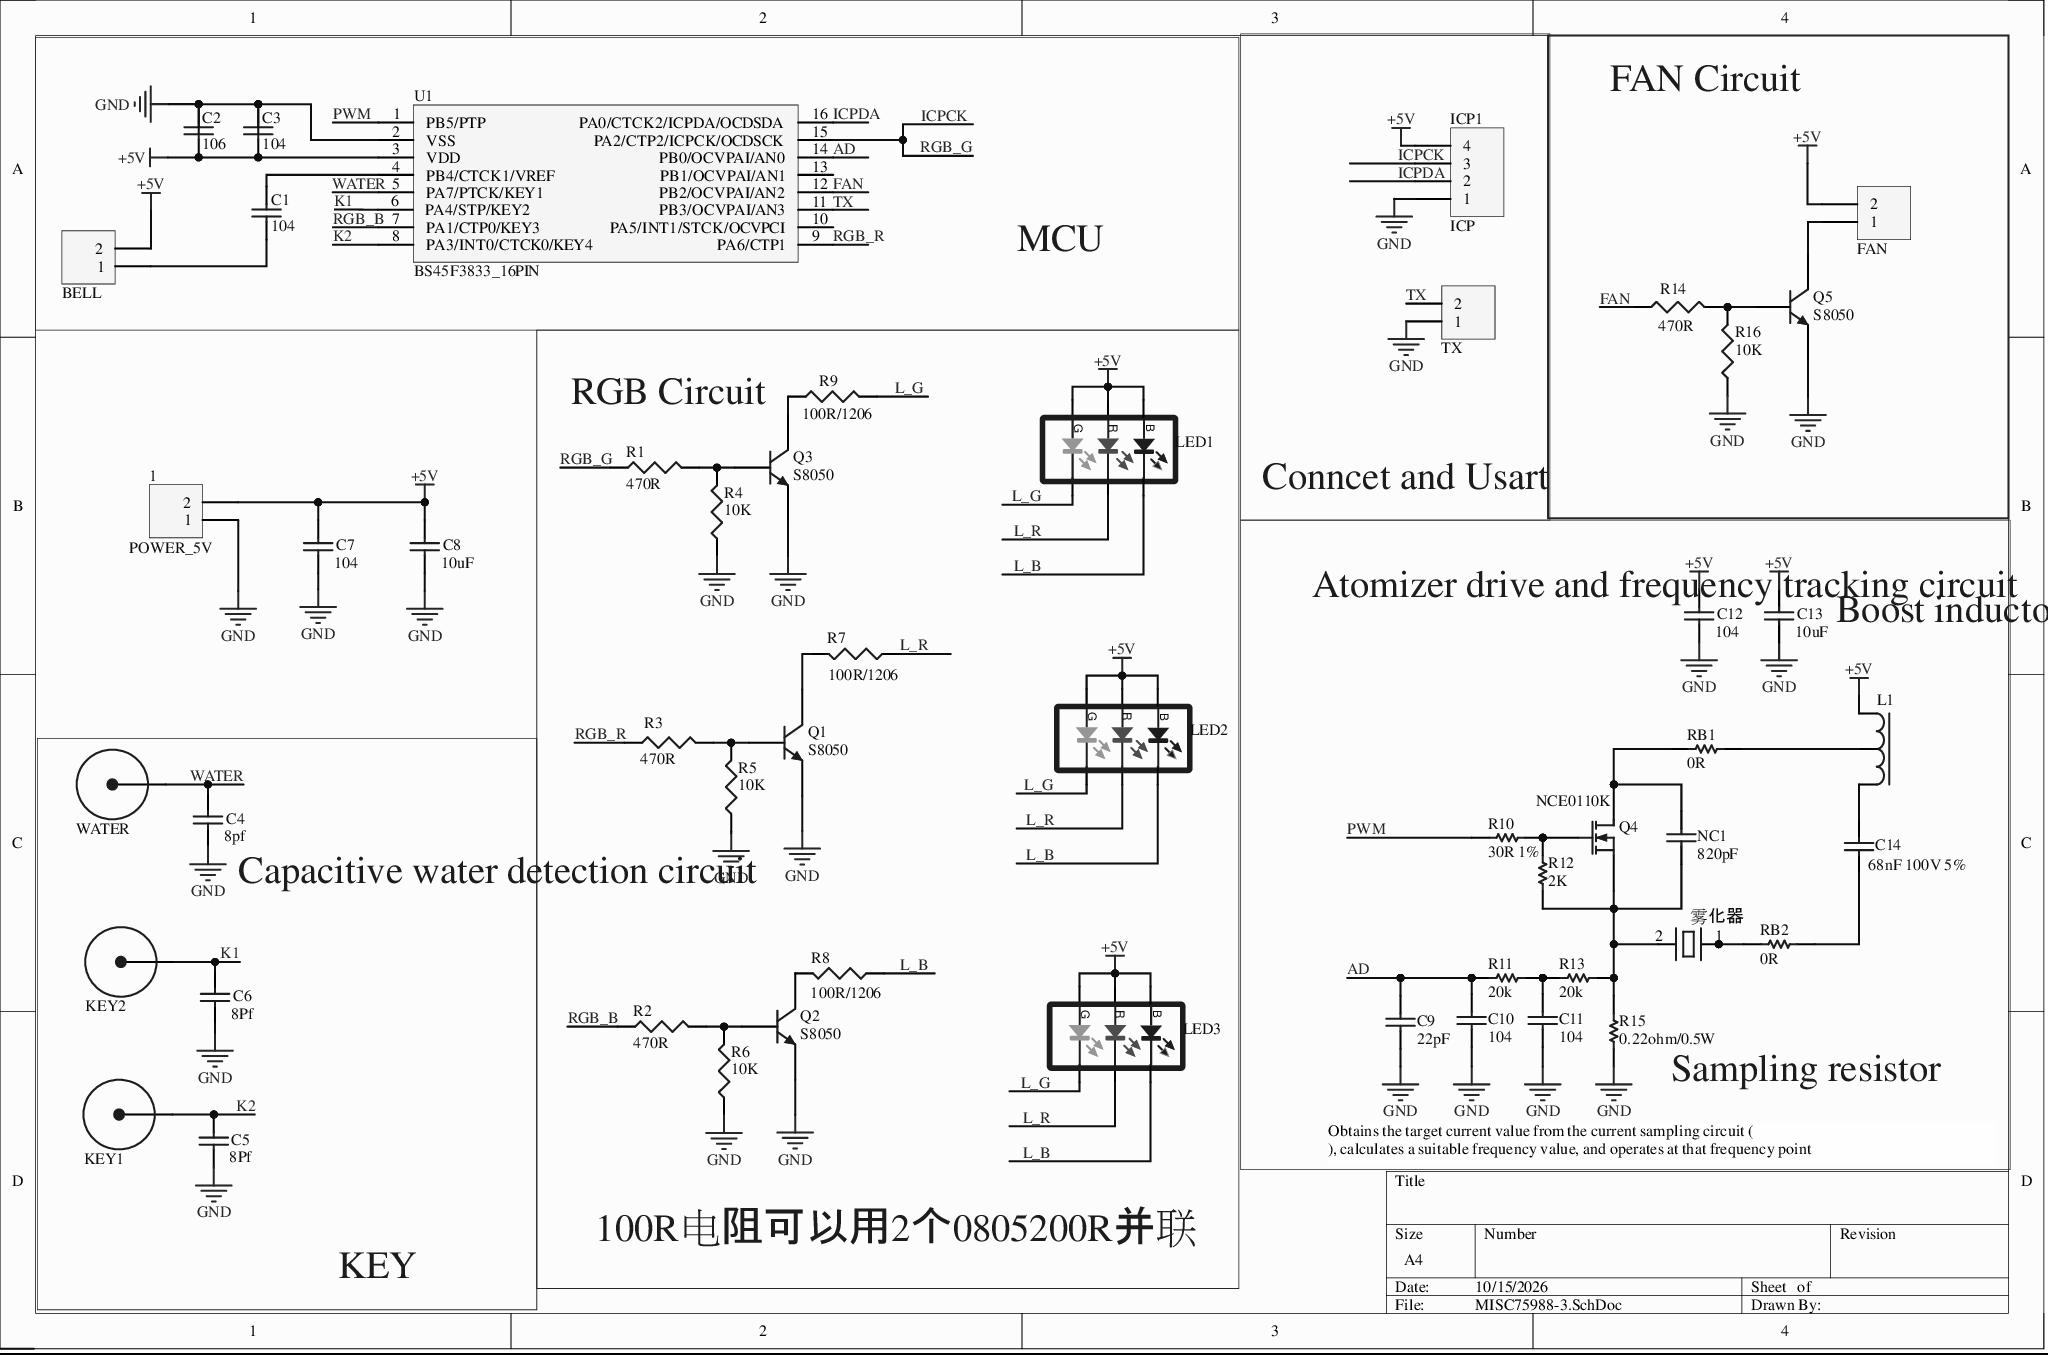
[diagram p0: MISC75988-3.SchDoc]
# Altium project MISC75988-6.PrjPcb
1 sheet, 52 parts. Net scope: global (net labels, ports and power ports of the same name join across sheets).
Board file: MISC75988.PcbDoc

## Sheet MISC75988-3.SchDoc
size A4; SheetNumber: 1; SheetTotal: 1

### Parts
1  POWER_5V  [con2-wafer]
BELL  BELL  [con2-wafer]
C1  value 104  [0603C]  (hidden comment: 0.1uF)
C2  value 106  [0603C]  (hidden comment: 0.1uF)
C3  value 104  [0603C]  (hidden comment: 0.1uF)
C4  value 8pf  [0603C]  (hidden comment: CAP)
C5  value 8Pf  [0603C]  (hidden comment: CAP)
C6  value 8Pf  [0603C]  (hidden comment: CAP)
C7  value 104  [0603C]  (hidden comment: CAP)
C8  value 10uF  [0603C]  (hidden comment: CAP)
C9  22pF  [0603C]
C10  value 104  [0603C]  (hidden comment: CAP)
C11  value 104  [0603C]  (hidden comment: CAP)
C12  value 104  [0603C]  (hidden comment: CAP)
C13  value 10uF  [0603C]  (hidden comment: CAP)
C14  value 68nF 100V 5%  [0603C]  (hidden comment: CAP)
FAN1  FAN  [con2-wafer]
ICP1  ICP  [HDR1X4]
KEY1  KEY1  [TP2]
KEY2  KEY2  [TP2]
L1  INDUCTOR  [TREE]  (value not drawn)
LED1  RGB  [LED-5050]  (value not drawn)
LED2  RGB  [LED-5050]  (value not drawn)
LED3  RGB  [LED-5050]  (value not drawn)
NC1  value 820pF  [0603C]  (hidden comment: CAP)
Q1  S8050  [SOT_23]
Q2  S8050  [SOT_23]
Q3  S8050  [SOT_23]
Q4  NCE0110K  [TO252-3]
Q5  S8050  [SOT_23]
R1  value 470R  [0603R]  (hidden comment: 2.2K)
R2  value 470R  [0603R]  (hidden comment: 2.2K)
R3  value 470R  [0603R]  (hidden comment: 15R)
R4  value 10K  [0603R]  (hidden comment: 2.2K)
R5  value 10K  [0603R]  (hidden comment: 2.2K)
R6  value 10K  [0603R]  (hidden comment: 2.2K)
R7  100R/1206  [0603R]
R8  100R/1206  [0603R]
R9  100R/1206  [0603R]
R10  value 30R 1%  [0603R]  (hidden comment: RES)
R11  value 20k  [0603R]  (hidden comment: RES)
R12  value 2K  [0603R]  (hidden comment: RES)
R13  value 20k  [0603R]  (hidden comment: RES)
R14  value 470R  [0603R]
R15  value 0.22ohm/0.5W  [2512]  (hidden comment: RES)
R16  value 10K  [0603R]  (hidden comment: 2.2K)
RB1  value 0R  [0603R]  (hidden comment: RES)
RB2  value 0R  [0603R]  (hidden comment: RES)
TX1  TX  [HDR1X2]
U1  BS45F3833_16PIN  [NSOP 16]
WATER1  WATER  [Touch-Pad]
雾化器  (no value)  [con2-wafer]

### Blocks framed on the sheet
Conncet and Usart: ICP1 TX1
MCU: BELL C1-C3 U1
FAN Circuit: FAN1 Q5 R14 R16

### Nets
+5V: 1.2 BELL.2 C2.1 C3.1 C7.2 C8.2 C12.2 C13.2 FAN1.2 ICP1.4 L1.1 LED1.1 LED1.2 LED1.3 LED2.1 LED2.2 LED2.3 LED3.1 LED3.2 LED3.3 U1.3(VDD)
GND: 1.1 C2.2 C3.2 C4.1 C5.1 C6.1 C7.1 C8.1 C9.1 C10.1 C11.1 C12.1 C13.1 ICP1.1 Q1.1(E) Q2.1(E) Q3.1(E) Q5.1(E) R4.1 R5.1 R6.1 R15.1 R16.1 TX1.1 U1.2(VSS)
AD: C9.2 C10.2 R11.1 U1.14(PB0/OCVPAI/AN0)
FAN: R14.1 U1.12(PB2/OCVPAI/AN2)
ICPCK: ICP1.3 R1.1 U1.15(PA2/CTP2/ICPCK/OCDSCK)  [also labelled RGB_G]
ICPDA: ICP1.2 U1.16(PA0/CTCK2/ICPDA/OCDSDA)
K1: C6.2 KEY2.1 U1.6(PA4/STP/KEY2)
K2: C5.2 KEY1.1 U1.8(PA3/INT0/CTCK0/KEY4)
L_B: LED1.6 LED2.6 LED3.6 R8.1
L_G: LED1.5 LED2.5 LED3.5 R9.2
L_R: LED1.4 LED2.4 LED3.4 R7.1
PWM: R10.1 U1.1(PB5/PTP)
RGB_B: R2.1 U1.7(PA1/CTP0/KEY3)
RGB_R: R3.1 U1.9(PA6/CTP1)
TX: TX1.2 U1.11(PB3/OCVPAI/AN3)
WATER: C4.2 U1.5(PA7/PTCK/KEY1) WATER1.1
NetBELL_1: BELL.1 C1.1
NetC1_2: C1.2 U1.4(PB4/CTCK1/VREF)
NetC11_2: C11.2 R11.2 R13.1
NetC14_1: C14.1 RB2.2
NetC14_2: C14.2 L1.3
NetFAN1_1: FAN1.1 Q5.3(C)
NetL1_2: L1.2 RB1.2
NetNC1_1: NC1.1 Q4.3(S) R12.1 R13.2 R15.2 雾化器.2(OSC2)
NetNC1_2: NC1.2 Q4.2(G) RB1.1
NetQ1_2: Q1.2(B) R3.2 R5.2
NetQ1_3: Q1.3(C) R7.2
NetQ2_2: Q2.2(B) R2.2 R6.2
NetQ2_3: Q2.3(C) R8.2
NetQ3_2: Q3.2(B) R1.2 R4.2
NetQ3_3: Q3.3(C) R9.1
NetQ4_1: Q4.1(D) R10.2 R12.2
NetQ5_2: Q5.2(B) R14.2 R16.2
NetRB2_1: RB2.1 雾化器.1(OSC1)

Not connected (* = marked no-connect by the designer): U1 10(PA5/INT1/STCK/OCVPCI)* 13(PB1/OCVPAI/AN1)*

### Notes on the sheet
- RGB Circuit
- Atomizer drive and frequency tracking circuit
- Boost inductor
- Capacitive water detection circuit
- (near R15) Sampling resistor
- Obtains the target current value from the current sampling circuit (
  ), calculates a suitable frequency value, and operates at that frequency point
- KEY
- 100R电阻可以用2个0805200R并联

### Library data of the parts
1 BELL FAN1 TX1 = Header 2: Header, 2-Pin; LatestRevisionDate: 17-Jul-2002; LatestRevisionNote: Re-released for DXP Platform.; Publisher: Altium Limited
C1-C3 = Cap: Capacitor; Published: 8-Jun-2000; LatestRevisionDate: 17-Jul-2002; LatestRevisionNote: Re-released for DXP Platform.; PackageReference: RAD-0.3; PackageDescription: Radial Cap, Thru-Hole; 2 Leads; 0.3 in Pin Spacing; Publisher: Altium Limited
C4-C14 NC1 = CAP_4: Published: 8-Jun-2000; LatestRevisionDate: 29-May-2009; LatestRevisionNote: IPC-7351 Footprint Added.; PackageReference: C1206; PackageDescription: Chip Capacitor; Publisher: Altium Limited
  C9: Value: 22pF
ICP1 = Header 4: Header, 4-Pin; LatestRevisionDate: 17-Jul-2002; LatestRevisionNote: Re-released for DXP Platform.; Publisher: Altium Limited
KEY1 KEY2 WATER1 = Touch-Pad
L1 = INDUCTOR5
LED1-LED3 = RGB-CREE(5)
Q1-Q3 Q5 = 2N3904: NPN General Purpose Amplifier; Published: 8-Jun-2000; LatestRevisionDate: 15-Jan-2003; LatestRevisionNote: PCB Footprint 'BCY-W3/D4.7' replaced; DatasheetVersion: 1997; PackageVersion: Sep-1998; PackageReference: TO-92A; PackageDescription: TO, Flat Index; 3 In-Line, Axial Leads; Body Dia. 4.5mm; Leads 0.51 x 0.48 mm (max); ComponentLink1Description: Manufacturer Link; ComponentLink2Description: Datasheet; ComponentLink2URL: http://www.fairchildsemi.com/ds/2N%2F2N3904.pdf; Publisher: Altium Limited
Q4 = MOSFET-N: N-Channel MOSFET; Published: 8-Jun-2000; LatestRevisionDate: 17-Jul-2002; LatestRevisionNote: Re-released for DXP Platform.; PackageVersion: 1995/1996; PackageReference: E3; PackageDescription: TO, Flat Index; 3 In-Line, Axial Leads; Body Dia. 4.6mm; Lead Dia. 0.5 mm (max); Publisher: Altium Limited
R1-R6 R14 R16 = Res3: Resistor; Published: 8-Jun-2000; LatestRevisionDate: 29-May-2009; LatestRevisionNote: IPC-7351 Footprint Added.; PackageReference: J1-0603; PackageDescription: Chip Resistor; Publisher: Altium Limited
R7 = Res3: Resistor; Value: 150R; Published: 8-Jun-2000; LatestRevisionDate: 29-May-2009; LatestRevisionNote: IPC-7351 Footprint Added.; PackageReference: J1-0603; PackageDescription: Chip Resistor; Publisher: Altium Limited
R8 = Res3: Resistor; Value: 120R; Published: 8-Jun-2000; LatestRevisionDate: 29-May-2009; LatestRevisionNote: IPC-7351 Footprint Added.; PackageReference: J1-0603; PackageDescription: Chip Resistor; Publisher: Altium Limited
R9 = Res3: Resistor; Value: 100R; Published: 8-Jun-2000; LatestRevisionDate: 29-May-2009; LatestRevisionNote: IPC-7351 Footprint Added.; PackageReference: J1-0603; PackageDescription: Chip Resistor; Publisher: Altium Limited
R10-R13 R15 RB1 RB2 = RES_4: Published: 8-Jun-2000; LatestRevisionDate: 17-Jul-2002; LatestRevisionNote: Re-released for DXP Platform.; PackageReference: AXIAL-0.3; PackageDescription: Axial Device, Thru-Hole; 2 Leads; 0.3 in Pin Spacing; Publisher: Altium Limited
雾化器 = CRYSTAL_1: Published: 8-Jun-2000; LatestRevisionDate: 17-Jul-2002; LatestRevisionNote: Re-released for DXP Platform.; PackageReference: R38; PackageDescription: Crystal, Thru-Hole; 2 Leads; Body 3.1 x 8.2 mm (Dia.xH); Publisher: Altium Limited